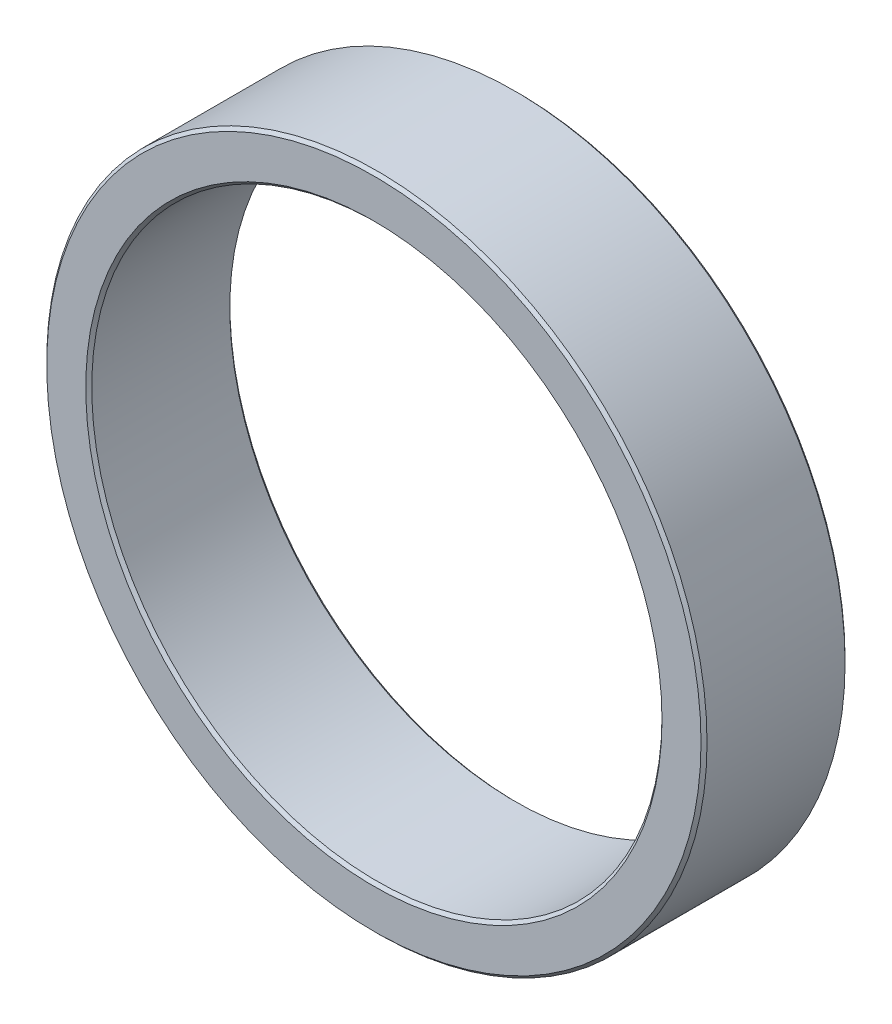
from build123d import *

# Parameters (mm, degrees)
SKETCH1_R           = 55
SKETCH1_R_2         = 47.5
BOSS_EXTRUDE1_DEPTH = 24
CHAMFER1_SIZE       = 0.5


with BuildPart() as part:
    # Sketch1 → Boss-Extrude1 (new body)
    with BuildSketch(Plane.XY):
        Circle(SKETCH1_R)
        Circle(SKETCH1_R_2, mode=Mode.SUBTRACT)
    extrude(amount=BOSS_EXTRUDE1_DEPTH)

    # Chamfer1
    chamfer1_edges = [part.edges().sort_by_distance(p)[0] for p in [
        (-55, 0, 0),
        (-55, 0, 24),
        (-47.5, 0, 0),
        (-47.5, 0, 24),
    ]]
    chamfer(chamfer1_edges, length=CHAMFER1_SIZE)


solid = part.part
